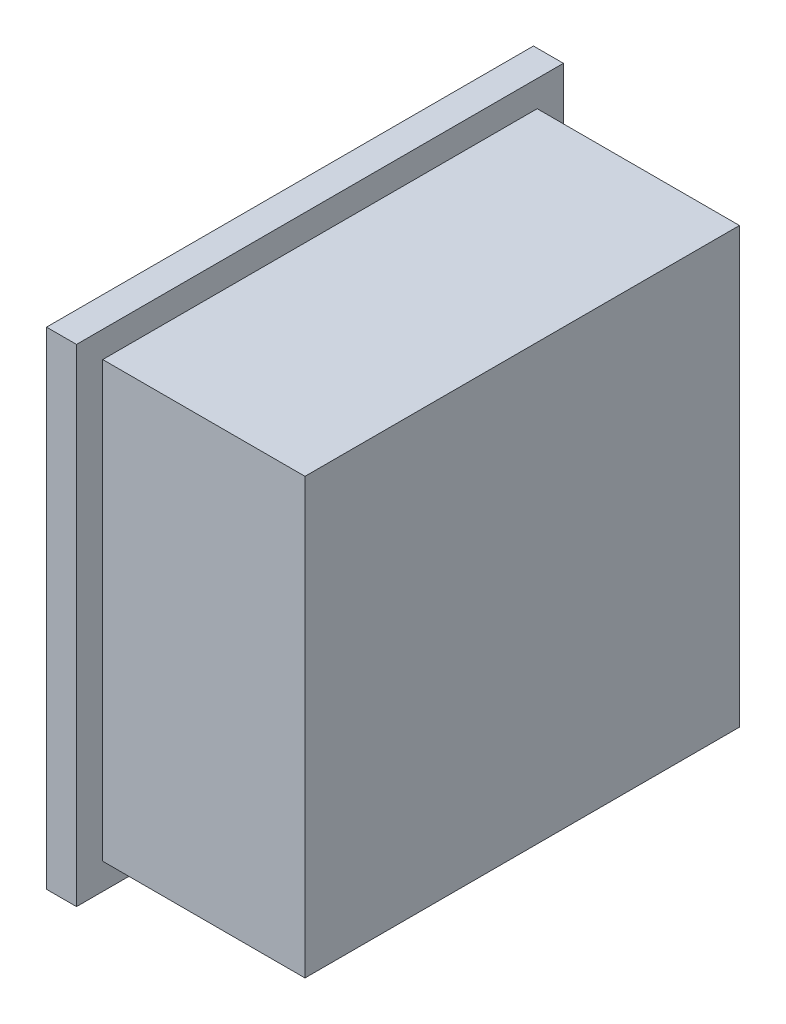
from build123d import *

# Parameters (mm, degrees)
SKETCH_1_W          = 130
SKETCH_1_H          = 130
EXTRUDE_1_DEPTH     = 8
SKETCH_2_W          = 116
SKETCH_2_H          = 116
EXTRUDE_2_DEPTH     = 54
SKETCH_3_W          = 114.015684478
SKETCH_3_H          = 114.394474128
CUT_EXTRUDE_1_DEPTH = 2


with BuildPart() as part:
    # 草图1 → 凸台-拉伸1 (new body)
    with BuildSketch(Plane(origin=(0, 0, 0), x_dir=(0, 0, -1), z_dir=(1, 0, 0))):
        Rectangle(SKETCH_1_W, SKETCH_1_H)
    extrude(amount=EXTRUDE_1_DEPTH)

    # 草图2 → 凸台-拉伸2 (add)
    with BuildSketch(Plane(origin=(8, 0, 0), x_dir=(0, 0, -1), z_dir=(1, 0, 0))):
        Rectangle(SKETCH_2_W, SKETCH_2_H)
    extrude(amount=EXTRUDE_2_DEPTH)

    # 草图3 → 切除-拉伸1 (cut)
    with BuildSketch(Plane.ZY):
        Rectangle(SKETCH_3_W, SKETCH_3_H)
    extrude(amount=-CUT_EXTRUDE_1_DEPTH, mode=Mode.SUBTRACT)


solid = part.part
